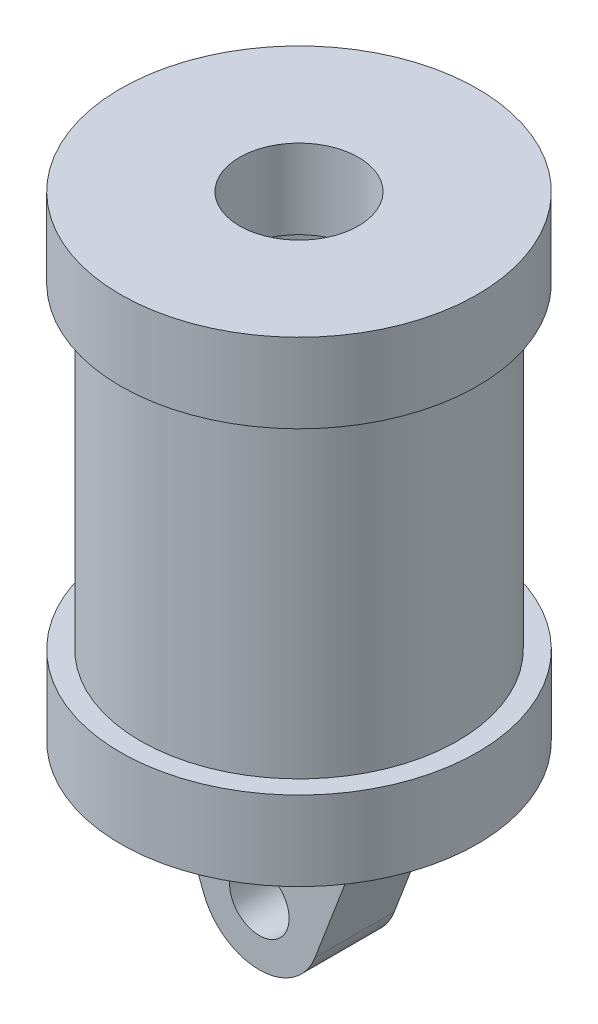
from build123d import *

# Parameters (mm, degrees)
SKETCH_1_R          = 40
EXTRUDE_1_DEPTH     = 80
SKETCH_2_R          = 45
EXTRUDE_2_DEPTH     = 20
EXTRUDE_START       = 20
SKETCH_3_R          = 45
EXTRUDE_3_DEPTH     = 20
CUT_EXTRUDE_START   = -20
SKETCH_4_R          = 30
CUT_EXTRUDE_2_DEPTH = 80
SKETCH_5_R          = 15
CUT_EXTRUDE_3_DEPTH = 40
SKETCH_6_R          = 7.5
EXTRUDE_4_DEPTH     = 10
FILLET_1_R          = 2


with BuildPart() as part:
    # 草图1 → 凸台-拉伸1 (new body)
    with BuildSketch(Plane(origin=(0, 0, 0), x_dir=(1, 0, 0), z_dir=(0, 1, 0))):
        with Locations(Location((0, 0, 0), (0, 0, 270))):
            Circle(SKETCH_1_R)
    extrude(amount=EXTRUDE_1_DEPTH)

    # 草图2 → 凸台-拉伸2 (add)
    with BuildSketch(Plane.XZ):
        with Locations(Location((0, 0, 0), (0, 0, 270))):
            Circle(SKETCH_2_R)
    extrude(amount=EXTRUDE_2_DEPTH)

    # 草图3 → 凸台-拉伸3 (add)
    with BuildSketch(Plane(origin=(0, 80, 0), x_dir=(1, 0, 0), z_dir=(0, 1, 0)).offset(EXTRUDE_START)):
        with Locations(Location((0, 0, 0), (0, 0, 90))):
            Circle(SKETCH_3_R)
    extrude(amount=-EXTRUDE_3_DEPTH)

    # 草图4 → 切除-拉伸2 (cut)
    with BuildSketch(Plane(origin=(0, 100, 0), x_dir=(1, 0, 0), z_dir=(0, 1, 0)).offset(CUT_EXTRUDE_START)):
        with Locations(Location((0, 0, 0), (0, 0, 270))):
            Circle(SKETCH_4_R)
    extrude(amount=-CUT_EXTRUDE_2_DEPTH, mode=Mode.SUBTRACT)

    # 草图5 → 切除-拉伸3 (cut)
    with BuildSketch(Plane(origin=(0, 100, 0), x_dir=(1, 0, 0), z_dir=(0, 1, 0))):
        with Locations(Location((0, 0, 0), (0, 0, 270))):
            Circle(SKETCH_5_R)
    extrude(amount=-CUT_EXTRUDE_3_DEPTH, mode=Mode.SUBTRACT)

    # 草图6 → 凸台-拉伸4 (add, symmetric)
    with BuildSketch(Plane.XY):
        with BuildLine():
            Line((-14.014695363, -55.346804082), (-27.5, -20))
            Line((-27.5, -20), (27.5, -20))
            Line((27.5, -20), (14.014695363, -55.346804082))
            ThreePointArc((14.014695363, -55.346804082), (0, -65), (-14.014695363, -55.346804082))
        make_face()
        with Locations((0, -50)):
            Circle(SKETCH_6_R, mode=Mode.SUBTRACT)
    extrude(amount=EXTRUDE_4_DEPTH, both=True)

    # 圆角1
    fillet_1_edges = [part.edges().sort_by_distance(p)[0] for p in [
        (0, -20, 10),
        (0, -20, -10),
        (27.5, -20, 0),
        (-27.5, -20, 0),
    ]]
    fillet(fillet_1_edges, radius=FILLET_1_R)


solid = part.part
